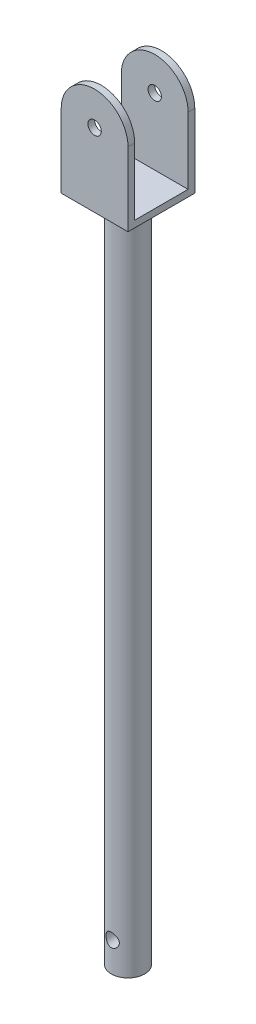
SolidWorks part; units mm, degrees
ref_plane "前视基准面" through (0, 0, 0) normal (0, 0, 1) x (1, 0, 0)
ref_plane "上视基准面" through (0, 0, 0) normal (0, 1, 0) x (1, 0, 0)
ref_plane "右视基准面" through (0, 0, 0) normal (1, 0, 0) x (0, 0, -1)
sketch "草图1" plane through (0, 0, 0) normal (0, 0, 1) x (1, 0, 0)
  line L0 (0, -29.9292) -> (0, 29.9292) construction
  line L1 (-10, 20) -> (-10, 0)
  line L2 (15.1151, 0) -> (-15.1151, 0) construction
  line L3 (-10, 0) -> (10, 0)
  line L4 (10, 0) -> (10, 20)
  arc A0 (10, 20) -> (-10, 20) centre (0, 20) ccw
  dimension "D1" = 20
  dimension "D2" = 20
extrude "凸台-拉伸1" add sketch "草图1" along normal mid plane 20
sketch "草图2" plane through (0, 0, -10) normal (0, 0, -1) x (-1, 0, 0)
  circle A0 centre (0, 20) radius 2
  dimension "D1" = 4
extrude "切除-拉伸1" cut sketch "草图2" against normal blind 34
sketch "草图3" plane through (0, 0, 0) normal (1, 0, 0) x (0, 0, -1)
  line L0 (-10, 30) -> (-10, 20) construction
  line L1 (-8, -43.9288) -> (8, -43.9288)
  line L2 (-8, -43.9288) -> (-8, 43.9288)
  line L3 (-8, 43.9288) -> (8, 43.9288)
  line L4 (8, -43.9288) -> (8, 43.9288)
  line L5 (-8, -43.9288) -> (8, 43.9288) construction
  line L6 (-8, 43.9288) -> (8, -43.9288) construction
  point P0 (0, 0)
  dimension "D1" = 2
extrude "切除-拉伸2" cut sketch "草图3" against normal mid plane 34
sketch "草图5" plane through (0, 0, 0) normal (0, -1, 0) x (1, 0, 0)
  line L1 (-10, -10) -> (10, -10)
  line L2 (-10, -10) -> (-10, 10)
  line L3 (-10, 10) -> (10, 10)
  line L4 (10, -10) -> (10, 10)
  line L5 (-10, -10) -> (10, 10) construction
  line L6 (-10, 10) -> (10, -10) construction
  point P0 (0, 0)
extrude "凸台-拉伸2" add sketch "草图5" along normal blind 2
sketch "草图6" plane through (0, -2, 0) normal (0, -1, 0) x (1, 0, 0)
  circle A0 centre (0, 0) radius 5
  dimension "D1" = 10
extrude "凸台-拉伸3" add sketch "草图6" along normal blind 200
sketch "草图7" plane through (0, 0, 0) normal (0, 0, 1) x (1, 0, 0)
  line L0 (0, -11) -> (0, 11) construction
  circle A0 centre (0, -193.1753) radius 2
  dimension "D1" = 4
extrude "切除-拉伸3" cut sketch "草图7" along normal mid plane 61
